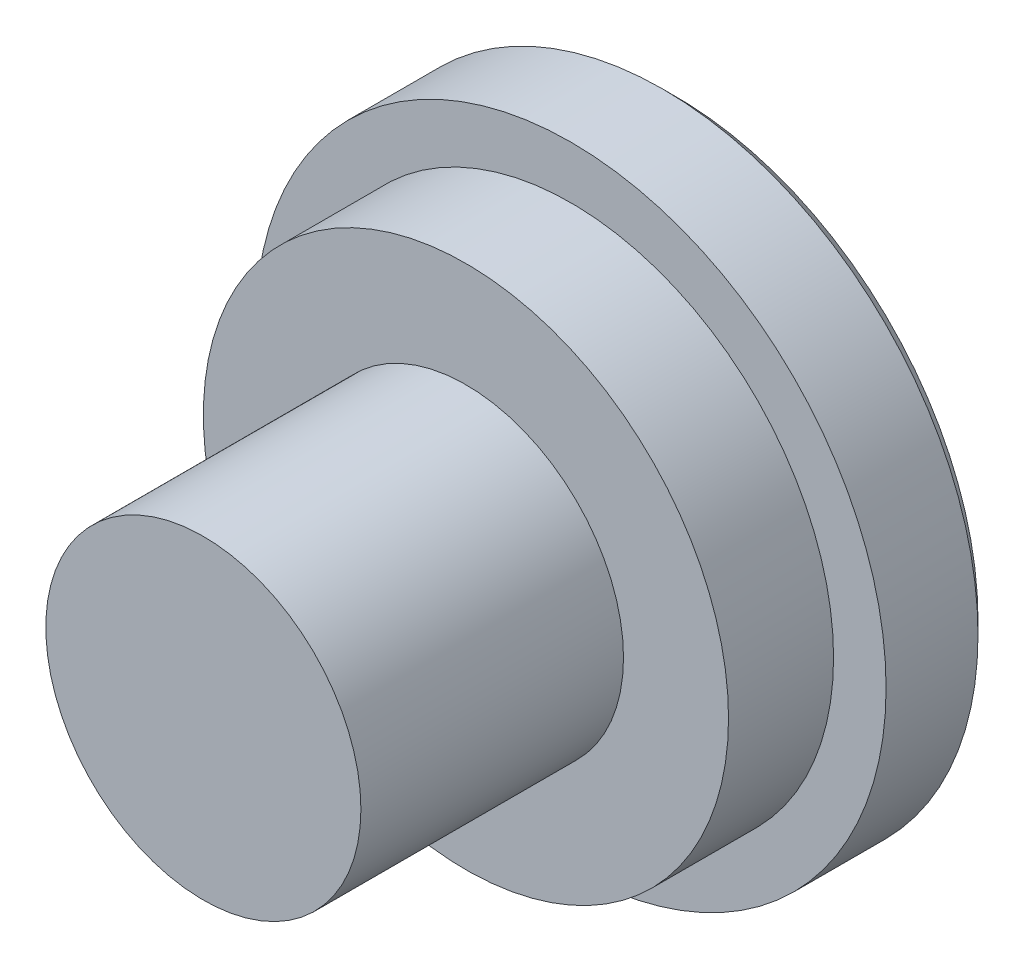
from build123d import *

# Parameters (mm, degrees)
SKETCH_1_4_R        = 6
BOSS_EXTRUDE1_DEPTH = 18
SKETCH_1_3_R        = 10
SKETCH_1_3_R_2      = 6
BOSS_EXTRUDE2_DEPTH = 8
SKETCH_1_4_2_R      = 12
SKETCH_1_4_2_R_2    = 10
BOSS_EXTRUDE3_DEPTH = 4
CHAMFER1_SIZE       = 0.5


with BuildPart() as part:
    # Sketch 1_4 → Boss-Extrude1 (new body)
    with BuildSketch(Plane.XY):
        Circle(SKETCH_1_4_R)
    extrude(amount=BOSS_EXTRUDE1_DEPTH)

    # 草图1<3> → Boss-Extrude2 (add)
    with BuildSketch(Plane.XY):
        Circle(SKETCH_1_3_R)
        Circle(SKETCH_1_3_R_2, mode=Mode.SUBTRACT)
    extrude(amount=BOSS_EXTRUDE2_DEPTH)

    # Sketch 1_4 2 → Boss-Extrude3 (add)
    with BuildSketch(Plane.XY):
        Circle(SKETCH_1_4_2_R)
        Circle(SKETCH_1_4_2_R_2, mode=Mode.SUBTRACT)
    extrude(amount=BOSS_EXTRUDE3_DEPTH)

    # Chamfer1
    chamfer1_edges = [part.edges().sort_by_distance(p)[0] for p in [
        (-12, 0, 0),
    ]]
    chamfer(chamfer1_edges, length=CHAMFER1_SIZE)


solid = part.part
